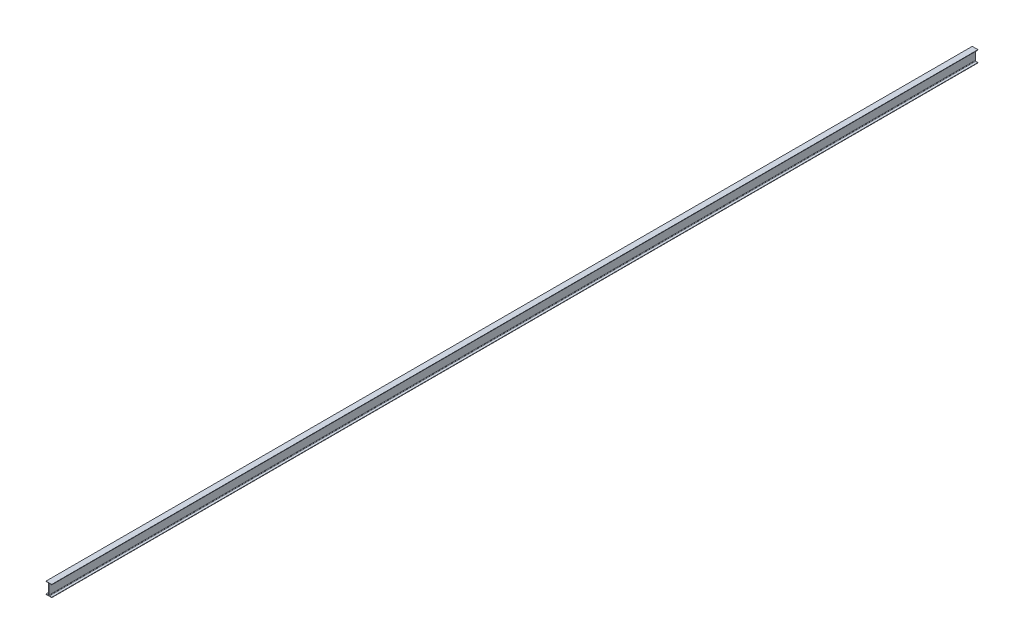
SolidWorks part; units mm, degrees
ref_plane "Front Plane" through (0, 0, 0) normal (0, 0, 1) x (1, 0, 0)
ref_plane "Top Plane" through (0, 0, 0) normal (0, 1, 0) x (1, 0, 0)
ref_plane "Right Plane" through (0, 0, 0) normal (1, 0, 0) x (0, 0, -1)
other "Configuration Table"
sketch "Sketch1" plane through (0, 0, 0) normal (0, 0, 1) x (1, 0, 0)
  line L0 (0, 0) -> (0, 300) construction
  line L1 (75, 0) -> (-75, 0)
  line L2 (-75, 0) -> (-75, 9)
  line L3 (-75, 9) -> (-16.25, 9)
  line L4 (3.25, 22) -> (3.25, 278)
  line L6 (-75, 291) -> (-75, 300)
  line L7 (-75, 300) -> (75, 300)
  line L8 (-3.25, 22) -> (-3.25, 278)
  line L9 (75, 291) -> (75, 300)
  line L10 (16.25, 291) -> (75, 291)
  line L11 (75, 9) -> (16.25, 9)
  line L12 (75, 0) -> (75, 9)
  line L13 (-16.25, 291) -> (-75, 291)
  arc A0 (16.25, 9) -> (3.25, 22) centre (16.25, 22) cw
  arc A1 (-3.25, 22) -> (-16.25, 9) centre (-16.25, 22) cw
  arc A2 (3.25, 278) -> (16.25, 291) centre (16.25, 278) cw
  arc A3 (-3.25, 278) -> (-16.25, 291) centre (-16.25, 278) ccw
  point P18 (3.25, 9)
  point P21 (-3.25, 9)
  point P24 (3.25, 291)
  point P27 (-3.25, 291)
  dimension "D6" = 13
  dimension "D1" = 300
  dimension "D2" = 150
  dimension "D3" = 6.5
  dimension "D4" = 9
  dimension "D5" = 9
extrude "Boss-Extrude1" add sketch "Sketch1" along normal blind 24174
